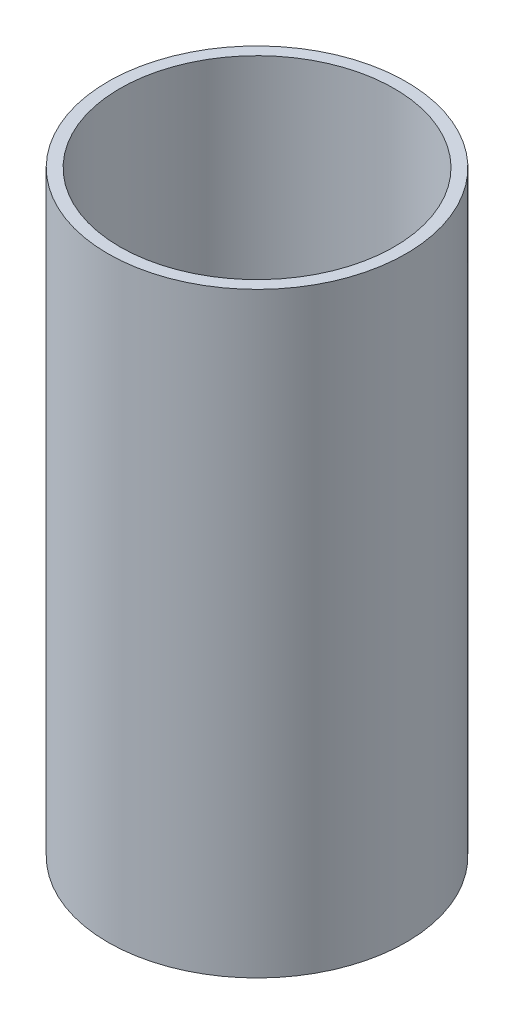
from build123d import *

# Parameters (mm, degrees)
SKETCH1_R           = 25
SKETCH1_R_2         = 23
BOSS_EXTRUDE1_DEPTH = 100


with BuildPart() as part:
    # Sketch1 → Boss-Extrude1 (new body)
    with BuildSketch(Plane(origin=(0, 0, 0), x_dir=(1, 0, 0), z_dir=(0, 1, 0))):
        with Locations(Location((0, 0, 0), (0, 0, 270))):
            Circle(SKETCH1_R)
        with Locations(Location((0, 0, 0), (0, 0, 270))):
            Circle(SKETCH1_R_2, mode=Mode.SUBTRACT)
    extrude(amount=BOSS_EXTRUDE1_DEPTH)


solid = part.part
